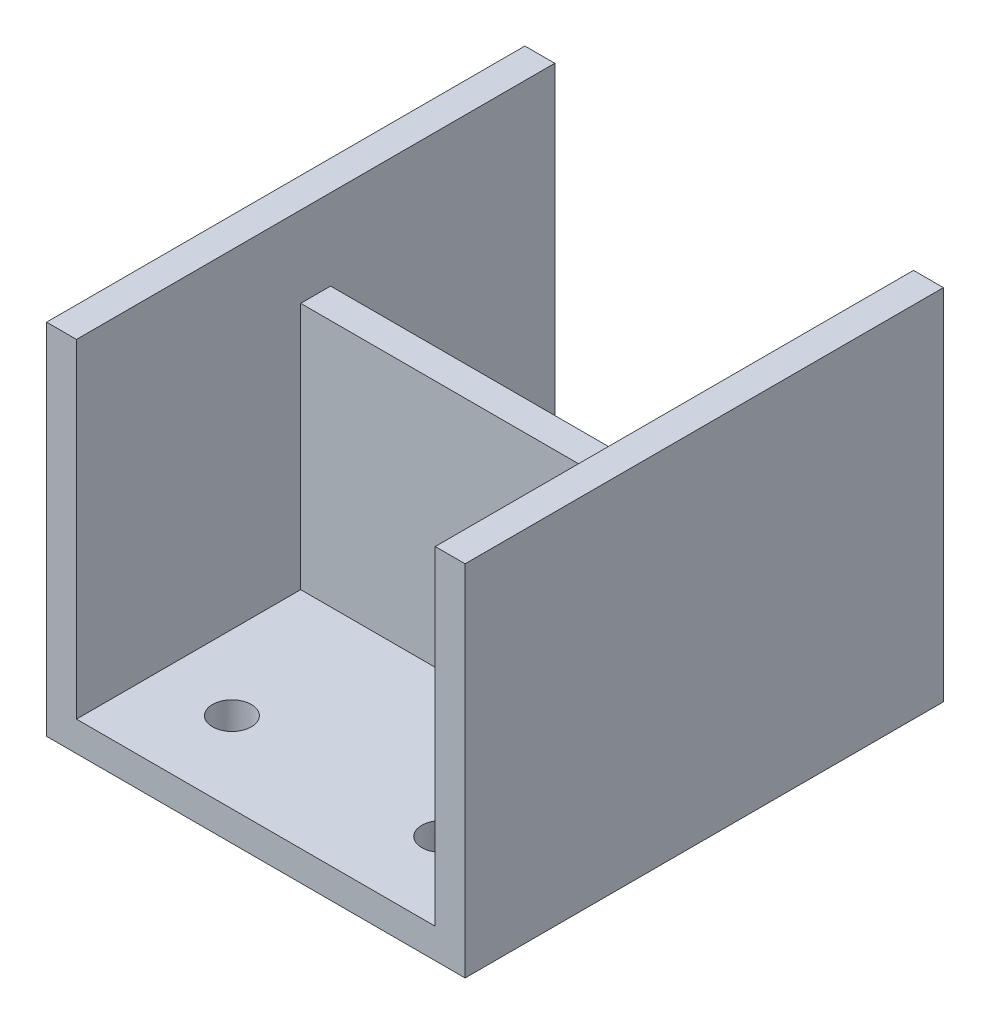
from build123d import *

# Parameters (mm, degrees)
EXTRUDE_1_DEPTH     = 40
SKETCH_2_W          = 60
SKETCH_2_H          = 41.476322839
EXTRUDE_2_DEPTH     = 2.5
SKETCH_3_R          = 3.25
CUT_EXTRUDE_1_DEPTH = 10


with BuildPart() as part:
    # 草图1 → 凸台-拉伸1 (new, symmetric)
    with BuildSketch(Plane.XY):
        Polygon((-30, 30), (-30, -25), (30, -25), (30, 30), (35, 30), (35, -30), (-35, -30), (-35, 30), align=None)
    extrude(amount=EXTRUDE_1_DEPTH, both=True)

    # 草图2 → 凸台-拉伸2 (add, symmetric)
    with BuildSketch(Plane.XY):
        with Locations((0, -4.26183858)):
            Rectangle(SKETCH_2_W, SKETCH_2_H)
    extrude(amount=EXTRUDE_2_DEPTH, both=True)

    # 草图3 → 切除-拉伸1 (cut)
    with BuildSketch(Plane.XZ.offset(30)):
        with Locations((17.5, 26.5)):
            Circle(SKETCH_3_R)
        with Locations((17.5, -8.5)):
            Circle(SKETCH_3_R)
        with Locations((-17.5, -8.5)):
            Circle(SKETCH_3_R)
        with Locations((-17.5, 26.5)):
            Circle(SKETCH_3_R)
    extrude(amount=-CUT_EXTRUDE_1_DEPTH, mode=Mode.SUBTRACT)


solid = part.part
